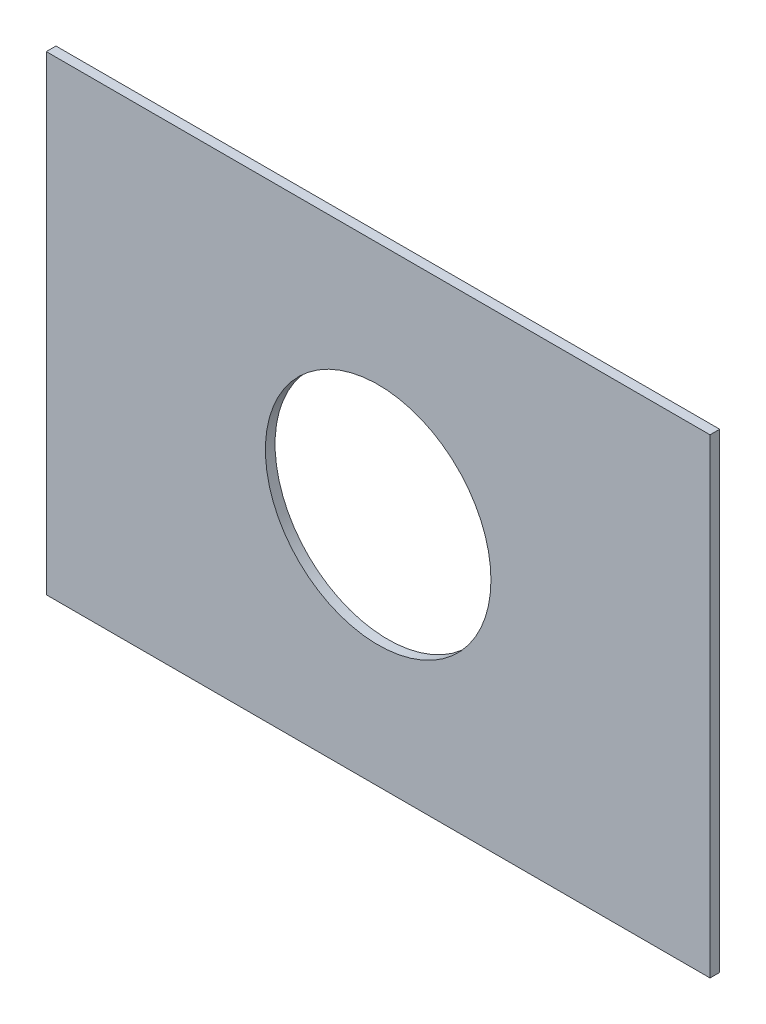
SolidWorks part; units mm, degrees
ref_plane "前视基准面" through (0, 0, 0) normal (0, 0, 1) x (1, 0, 0)
ref_plane "上视基准面" through (0, 0, 0) normal (0, 1, 0) x (1, 0, 0)
ref_plane "右视基准面" through (0, 0, 0) normal (1, 0, 0) x (0, 0, -1)
other "Configuration Table"
sketch "草图1" plane through (0, 0, 0) normal (0, 0, 1) x (1, 0, 0)
  line L0 (-103, -73) -> (103, -73)
  line L1 (103, -73) -> (103, 73)
  line L2 (103, 73) -> (-103, 73)
  line L3 (-103, 73) -> (-103, -73)
  point P0 (0, 0)
  dimension "D1" = 103
  dimension "D2" = 206
  dimension "D3" = 73
  dimension "D4" = 146
extrude "凸台-拉伸1" add sketch "草图1" against normal mid plane 3
sketch "草图2" plane through (0, 0, 0) normal (0, 0, 1) x (1, 0, 0)
  circle A0 centre (0, 0) radius 35
  point P0 (0, 0)
  dimension "D1" = 70
extrude "切除-拉伸1" cut sketch "草图2" against normal mid plane 23
